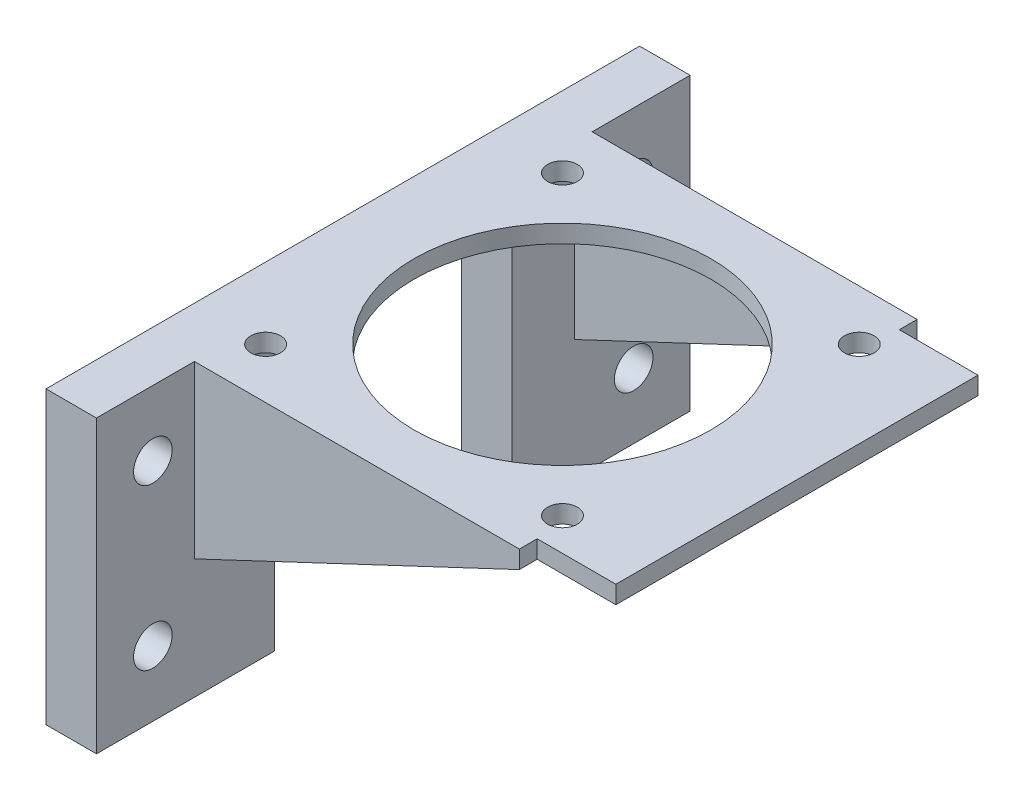
SolidWorks part; units mm, degrees
ref_plane "前视基准面" through (0, 0, 0) normal (0, 0, 1) x (1, 0, 0)
ref_plane "上视基准面" through (0, 0, 0) normal (0, 1, 0) x (1, 0, 0)
ref_plane "右视基准面" through (0, 0, 0) normal (1, 0, 0) x (0, 0, -1)
sketch "草图1" plane through (0, 0, 0) normal (1, 0, 0) x (0, 0, -1)
  line L1 (50, -24.5) -> (-50, -24.5)
  line L2 (50, -24.5) -> (50, 24.5)
  line L3 (50, 24.5) -> (-50, 24.5)
  line L4 (-50, -24.5) -> (-50, 24.5)
  line L5 (50, -24.5) -> (-50, 24.5) construction
  line L6 (50, 24.5) -> (-50, -24.5) construction
  line L7 (40.5, -13.5) -> (-40.5, -13.5) construction
  line L8 (40.5, -13.5) -> (40.5, 13.5) construction
  line L9 (40.5, 13.5) -> (-40.5, 13.5) construction
  line L10 (-40.5, -13.5) -> (-40.5, 13.5) construction
  line L11 (40.5, -13.5) -> (-40.5, 13.5) construction
  line L12 (40.5, 13.5) -> (-40.5, -13.5) construction
  circle A0 centre (-40.5, 13.5) radius 3.25
  circle A1 centre (40.5, 13.5) radius 3.25
  circle A2 centre (40.5, -13.5) radius 3.25
  circle A3 centre (-40.5, -13.5) radius 3.25
  point P0 (0, 0)
  point P6 (0, 0)
  dimension "D5" = 6.5
  dimension "D1" = 49
  dimension "D2" = 100
  dimension "D3" = 27
  dimension "D4" = 81
extrude "凸台-拉伸1" add sketch "草图1" along normal blind 8.5
sketch "草图2" plane through (8.5, 0, 0) normal (1, 0, 0) x (0, 0, -1)
  line L0 (50, 24.5) -> (-50, 24.5) construction
  line L1 (30.5, 21.5) -> (-30.5, 21.5)
  line L2 (30.5, 21.5) -> (30.5, 24.5)
  line L3 (30.5, 24.5) -> (-30.5, 24.5)
  line L4 (-30.5, 21.5) -> (-30.5, 24.5)
  line L5 (30.5, 21.5) -> (-30.5, 24.5) construction
  line L6 (30.5, 24.5) -> (-30.5, 21.5) construction
  line L7 (0, 23) -> (0, 0) construction
  point P0 (0, 23)
  dimension "D1" = 3
  dimension "D2" = 61
extrude "凸台-拉伸2" add sketch "草图2" along normal blind 68
sketch "草图3" plane through (0, 21.5, 0) normal (0, -1, 0) x (1, 0, 0)
  line L0 (37, 0) -> (76.5, 0) construction
  line L1 (76.5, 30.5) -> (76.5, -30.5) construction
  line L2 (0, 50) -> (0, -50) construction
  circle A0 centre (37, 0) radius 25
  dimension "D1" = 37
  dimension "D2" = 50
extrude "切除-拉伸1" cut sketch "草图3" against normal blind 68
sketch "草图4" plane through (0, 21.5, 0) normal (0, -1, 0) x (1, 0, 0)
  line L1 (62, -25) -> (12, -25) construction
  line L2 (62, -25) -> (62, 25) construction
  line L3 (62, 25) -> (12, 25) construction
  line L4 (12, -25) -> (12, 25) construction
  line L5 (62, -25) -> (12, 25) construction
  line L6 (62, 25) -> (12, -25) construction
  circle A0 centre (12, 25) radius 2.5
  circle A1 centre (62, 25) radius 2.5
  circle A2 centre (62, -25) radius 2.5
  circle A3 centre (12, -25) radius 2.5
  point P0 (37, 0)
  dimension "D3" = 5
  dimension "D1" = 50
  dimension "D2" = 50
extrude "切除-拉伸2" cut sketch "草图4" against normal blind 68
sketch "草图5" plane through (8.5, 0, 0) normal (1, 0, 0) x (0, 0, -1)
  line L0 (-30.5, 21.5) -> (30.5, 21.5) construction
  line L1 (20, -24.5) -> (-20, -24.5)
  line L2 (20, -24.5) -> (20, 21.5)
  line L3 (20, 21.5) -> (-20, 21.5)
  line L4 (-20, -24.5) -> (-20, 21.5)
  line L5 (20, -24.5) -> (-20, 21.5) construction
  line L6 (20, 21.5) -> (-20, -24.5) construction
  line L7 (0, -1.5) -> (0, -24.5) construction
  line L8 (-50, -24.5) -> (50, -24.5) construction
  point P0 (0, -1.5)
  dimension "D1" = 40
extrude "切除-拉伸3" cut sketch "草图5" against normal blind 15
sketch "草图6" plane through (0, 0, -30.5) normal (0, 0, -1) x (-1, 0, 0)
  line L0 (-63.2402, 24.5) -> (-63.2402, 21.5)
  line L1 (-76.5, 24.5) -> (-8.5, 24.5) construction
  line L2 (-76.5, 21.5) -> (-8.5, 21.5) construction
  line L3 (-63.2402, 21.5) -> (-8.5, -4.299)
  line L4 (-8.5, -24.5) -> (-8.5, 24.5) construction
  line L5 (-8.5, -4.299) -> (-8.5, 24.5)
  line L6 (-8.5, 24.5) -> (-63.2402, 24.5)
extrude "凸台-拉伸3" add sketch "草图6" along normal blind 3
mirror "镜向1" about plane through (0, 0, 0) normal (0, 0, 1) of "凸台-拉伸3"
